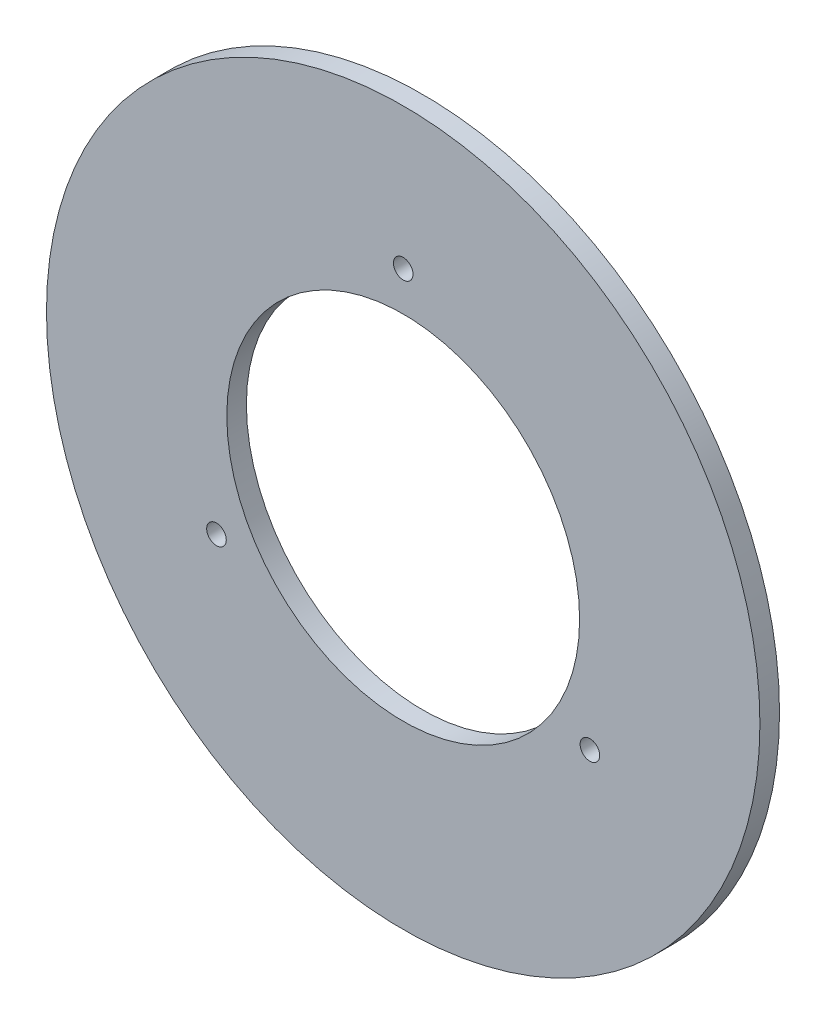
SolidWorks part; units mm, degrees
ref_plane "Front Plane" through (0, 0, 0) normal (0, 0, 1) x (1, 0, 0)
ref_plane "Top Plane" through (0, 0, 0) normal (0, 1, 0) x (1, 0, 0)
ref_plane "Right Plane" through (0, 0, 0) normal (1, 0, 0) x (0, 0, -1)
sketch "Sketch1" plane through (0, 0, 0) normal (0, 0, 1) x (1, 0, 0)
  circle A0 centre (0, 0) radius 91
  circle A1 centre (0, 0) radius 45
  circle A2 centre (0, 0) radius 55 construction
  circle A3 centre (0, 55) radius 2.5
  circle A4 centre (47.6314, -27.5) radius 2.5
  circle A5 centre (-47.6314, -27.5) radius 2.5
  point P14 (0, 0)
  dimension "D1" = 90
  dimension "D2" = 182
  dimension "D3" = 110
  dimension "D4" = 5
  dimension "D5" = 3
extrude "Boss-Extrude1" add sketch "Sketch1" along normal blind 5
